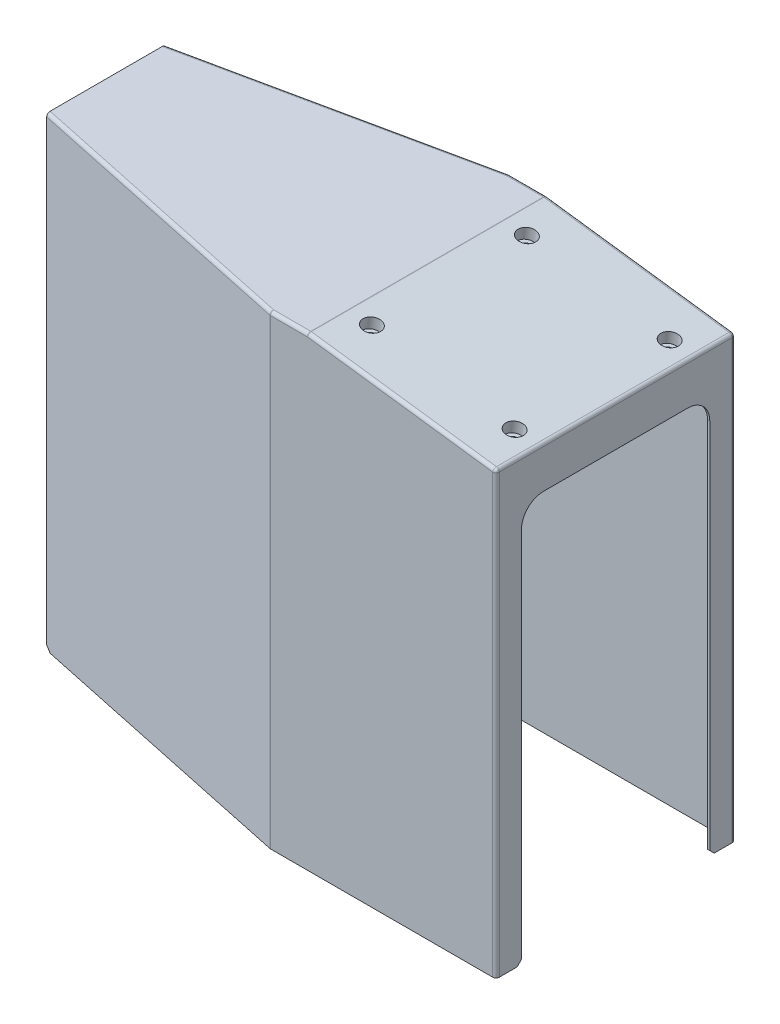
from build123d import *

# Parameters (mm, degrees)
SKETCH1_W                                            = 230
SKETCH1_H                                            = 108
BOSS_EXTRUDE1_DEPTH                                  = 105
CUT_EXTRUDE1_DEPTH                                   = 246.440420469
CUT_EXTRUDE2_DEPTH                                   = 190.509894201
FILLET1_R                                            = 1.5
SHELL1_T                                             = -1
SKETCH4_R                                            = 6
BOSS_EXTRUDE2_DEPTH                                  = 7
HOLE_SIZE_PER_SOCKET_HEAD_CAP_SCREW_TYPE_D           = 4.5
HOLE_SIZE_PER_SOCKET_HEAD_CAP_SCREW_TYPE_CBORE_D     = 8
HOLE_SIZE_PER_SOCKET_HEAD_CAP_SCREW_TYPE_CBORE_DEPTH = 5
CUT_EXTRUDE3_REACH                                   = 260.536
CHAMFER1_SIZE                                        = 2


with BuildPart() as part:
    # Sketch1 → Boss-Extrude1 (new, symmetric)
    with BuildSketch(Plane(origin=(0, 0, 0), x_dir=(1, 0, 0), z_dir=(0, 1, 0))):
        Rectangle(SKETCH1_W, SKETCH1_H)
    extrude(amount=BOSS_EXTRUDE1_DEPTH, both=True)

    # Sketch2 → Cut-Extrude1 (cut, through all)
    with BuildSketch(Plane(origin=(0, 105, 0), x_dir=(1, 0, 0), z_dir=(0, 1, 0))):
        Polygon((-115, 26.839455747), (-115, 54), (13, 54), align=None)
        Polygon((-115, -26.839455747), (-115, -54), (13, -54), align=None)
    extrude(amount=-CUT_EXTRUDE1_DEPTH, mode=Mode.SUBTRACT)

    # Sketch3 → Cut-Extrude2 (cut, through all)
    with BuildSketch(Plane.XY.offset(54)):
        Polygon((30, 105), (115, 105), (115, 93.809537705), align=None)
    extrude(amount=-CUT_EXTRUDE2_DEPTH, mode=Mode.SUBTRACT)

    # Fillet1
    fillet1_edges = [part.edges().sort_by_distance(p)[0] for p in [
        (13, 0, -54),
        (-51, 105, -40.419727874),
        (21.5, 105, 54),
        (13, 0, 54),
        (-51, 105, 40.419727874),
        (21.5, 105, -54),
        (115, -5.595231147, 54),
        (115, -5.595231147, -54),
        (72.5, 99.404768853, -54),
        (115, 93.809537705, 0),
        (30, 105, 0),
        (72.5, 99.404768853, 54),
    ]]
    fillet(fillet1_edges, radius=FILLET1_R)

    # Shell1
    shell1_openings = [part.faces().sort_by_distance(p)[0] for p in [
        (11.766407096, -105, 0),
        (-115, -0.009166967, 0),
    ]]
    offset(amount=SHELL1_T, openings=shell1_openings, kind=Kind.INTERSECTION)

    # Sketch4 → Boss-Extrude2 (add)
    with BuildSketch(Plane(origin=(13.968586281, 106.101946695, 0), x_dir=(0.9914448613738114, -0.1305261922200448, 0), z_dir=(-0.1305261922200448, -0.9914448613738114, 0))):
        with Locations((26.071147756, 35)):
            Circle(SKETCH4_R)
        with Locations((26.071147756, -35)):
            Circle(SKETCH4_R)
        with Locations((91.071147756, -35)):
            Circle(SKETCH4_R)
        with Locations((91.071147756, 35)):
            Circle(SKETCH4_R)
    extrude(amount=BOSS_EXTRUDE2_DEPTH)

    # Hole size per socket head cap screw type1 (through all)
    with Locations(Plane(origin=(14.099112474, 107.093391557, 0), x_dir=(0.9914448613738114, -0.1305261922200448, 0), z_dir=(0.1305261922200448, 0.9914448613738114, 0))):
        with Locations((26.071147756, 35), (91.071147756, 35), (91.071147756, -35), (26.071147756, -35)):
            CounterBoreHole(HOLE_SIZE_PER_SOCKET_HEAD_CAP_SCREW_TYPE_D / 2, HOLE_SIZE_PER_SOCKET_HEAD_CAP_SCREW_TYPE_CBORE_D / 2, HOLE_SIZE_PER_SOCKET_HEAD_CAP_SCREW_TYPE_CBORE_DEPTH)

    # Sketch7 → Cut-Extrude3 (cut, up to next)
    with BuildSketch(Plane(origin=(115, 0, 0), x_dir=(0, 0, -1), z_dir=(1, 0, 0)), mode=Mode.PRIVATE) as cut_extrude3_sk1:
        with BuildLine():
            Line((-42.5, -105), (42.5, -105))
            Line((42.5, -105), (42.5, 65))
            ThreePointArc((42.5, 65), (39.571067812, 72.071067812), (32.5, 75))
            Line((32.5, 75), (-32.5, 75))
            ThreePointArc((-32.5, 75), (-39.571067812, 72.071067812), (-42.5, 65))
            Line((-42.5, 65), (-42.5, -105))
        make_face()
    cut_extrude3_tool1 = extrude(cut_extrude3_sk1.sketch, amount=-CUT_EXTRUDE3_REACH, mode=Mode.PRIVATE) & part.part
    add(cut_extrude3_tool1.solids().sort_by_distance((115, -15.246899, 0))[0], mode=Mode.SUBTRACT)

    # Chamfer1
    chamfer1_edges = [part.edges().sort_by_distance(p)[0] for p in [
        (-115, -105, -26.328323343),
        (114.5, -105, 42.5),
        (114.5, -105, -42.5),
        (-115, -105, 26.328323343),
    ]]
    chamfer(chamfer1_edges, length=CHAMFER1_SIZE)


solid = part.part
